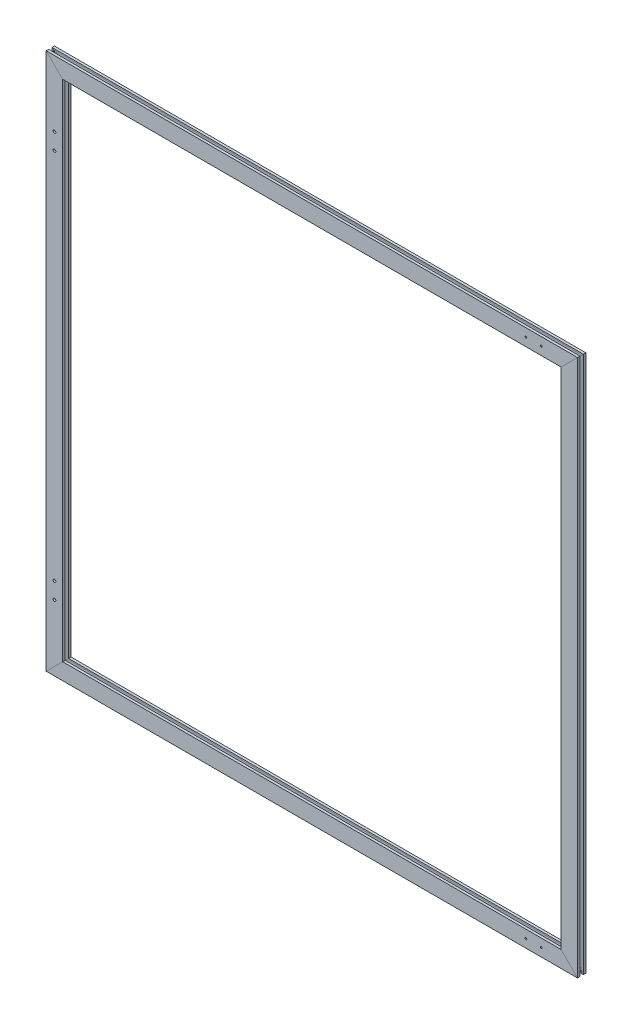
SolidWorks part; units mm, degrees
ref_plane "Front" through (0, 0, 0) normal (0, 0, 1) x (1, 0, 0)
ref_plane "Top" through (0, 0, 0) normal (0, 1, 0) x (1, 0, 0)
ref_plane "Right" through (0, 0, 0) normal (1, 0, 0) x (0, 0, -1)
sketch3d "3DSketch1"
  line L1 (468.5, 474, 0) -> (-468.5, 474, 0)
  line L2 (468.5, 474, 0) -> (468.5, -474, 0)
  line L3 (468.5, -474, 0) -> (-468.5, -474, 0)
  line L4 (-468.5, 474, 0) -> (-468.5, -474, 0)
  line L5 (468.5, 474, 0) -> (-468.5, -474, 0) construction
  line L6 (468.5, -474, 0) -> (-468.5, 474, 0) construction
  point P0 (0, 0, 0)
  dimension "D1" = 937
  dimension "D2" = 948
other "Aluminum profile 1530(1)"
ref_plane "Plane1" through (-468.5, 474, 0) normal (0, -1, 0) x (1, 0, 0)
sketch "Sketch1" plane through (-468.5, 474, 0) normal (0, -1, 0) x (1, 0, 0)
  line L4 (-15, -3) -> (-15, -7.5)
  line L5 (-15, -3) -> (-12.5, -3)
  line L6 (-15, -7.5) -> (15, -7.5)
  line L7 (-12.5, -3) -> (-12.5, -5)
  line L8 (15, -3) -> (15, -7.5)
  line L9 (-12.5, -5) -> (-7, -5)
  line L10 (15, -3) -> (12.5, -3)
  line L11 (-7, -5) -> (-7, -3)
  line L12 (12.5, -3) -> (12.5, -5)
  line L13 (-7, -3) -> (-4.5, -3)
  line L14 (12.5, -5) -> (7, -5)
  line L15 (-4.5, -3) -> (-4.5, 3)
  line L16 (7, -5) -> (7, -3)
  line L17 (-4.5, 3) -> (-7, 3)
  line L18 (7, -3) -> (4.5, -3)
  line L19 (-7, 3) -> (-7, 5)
  line L20 (4.5, -3) -> (4.5, 3)
  line L21 (-7, 5) -> (-12.5, 5)
  line L22 (4.5, 3) -> (7, 3)
  line L23 (-12.5, 5) -> (-12.5, 3)
  line L24 (7, 3) -> (7, 5)
  line L25 (-12.5, 3) -> (-15, 3)
  line L26 (7, 5) -> (12.5, 5)
  line L27 (-15, 7.5) -> (-15, 3)
  line L28 (12.5, 5) -> (12.5, 3)
  line L29 (15, 7.5) -> (-15, 7.5)
  line L30 (12.5, 3) -> (15, 3)
  line L31 (15, 7.5) -> (15, 3)
  circle A0 centre (0, 0) radius 2.5
  point P0 (0, 0)
other "Trim/Extend1"
other "Trim/Extend2"
other "Trim/Extend3"
other "Trim/Extend4"
hole_wizard "M6 Tapped Hole1" positions "Sketch4" profile "Sketch5" tap size "M6" standard "GB" end condition through all
sketch "Sketch4" plane through (0, 0, 7.5) normal (0, 0, 1) x (1, 0, 0)
  line L0 (-468.5, 369) -> (-468.5, 339)
  line L1 (-468.5, 339) -> (-468.5, -339)
  line L2 (-468.5, -339) -> (-468.5, -369)
  line L4 (-468.5, 0) -> (0, 0)
  line L5 (-483.5, 489) -> (483.5, 489) construction
  line L6 (-483.5, -489) -> (-483.5, 489) construction
  point P0 (-468.5, 369)
  point P2 (-468.5, 339)
  point P4 (-468.5, -339)
  point P6 (-468.5, -369)
  dimension "D1" = 120
  dimension "D2" = 15
  dimension "D3" = 30
sketch "Sketch5" plane through (-468.5, 369, 7.5) normal (1, 0, 0) x (0, -1, 0)
  line L0 (0, 0) -> (0, 15)
  line L1 (0, 15) -> (2.5, 15)
  line L2 (2.5, 15) -> (2.5, 0)
  line L5 (2.5, 0) -> (0, 0)
  line L11 (0, -6.35) -> (0, 107.95) construction
  dimension "通孔螺纹孔钻头直径" = 5
  dimension "通孔螺纹孔钻头深度" = 15
cosmetic thread "Hole-Thread1" parameters "D2"=6
cosmetic thread "Hole-Thread2" parameters "D2"=6
cosmetic thread "Hole-Thread3" parameters "D2"=6
cosmetic thread "Hole-Thread4" parameters "D2"=6
hole_wizard "M4 Tapped Hole1" positions "Sketch6" profile "Sketch7" tap size "M4" standard "GB"
sketch "Sketch6" plane through (0, 0, 7.5) normal (0, 0, 1) x (1, 0, 0)
  line L1 (389.5, -474) -> (417.5, -474)
  line L2 (389.5, -474) -> (389.5, 474)
  line L3 (389.5, 474) -> (417.5, 474)
  line L4 (417.5, -474) -> (417.5, 474)
  line L5 (-483.5, -489) -> (483.5, -489) construction
  line L6 (417.5, 0) -> (483.5, 0)
  line L7 (483.5, -489) -> (483.5, 489) construction
  point P0 (389.5, 474)
  point P2 (417.5, 474)
  point P4 (389.5, -474)
  point P6 (417.5, -474)
  point P66 (403.5, 474)
  dimension "D1" = 28
  dimension "D2" = 15
  dimension "D3" = 80
sketch "Sketch7" plane through (389.5, 474, 7.5) normal (1, 0, 0) x (0, -1, 0)
  line L0 (0, 0) -> (0, 12.4914)
  line L1 (0, 12.4914) -> (1.65, 11.5)
  line L2 (1.65, 11.5) -> (1.65, 0)
  line L5 (1.65, 0) -> (0, 0)
  line L10 (0, 12.4914) -> (-1.65, 11.5) construction
  line L11 (0, -6.35) -> (0, 107.95) construction
  dimension "螺纹孔钻头直径" = 3.3
  dimension "螺纹孔钻头深度" = 11.5
  dimension "导头角度" = 118
cosmetic thread "Hole-Thread5" parameters "D1"=8, "D2"=4
cosmetic thread "Hole-Thread6" parameters "D1"=8, "D2"=4
cosmetic thread "Hole-Thread7" parameters "D1"=8, "D2"=4
cosmetic thread "Hole-Thread8" parameters "D1"=8, "D2"=4
